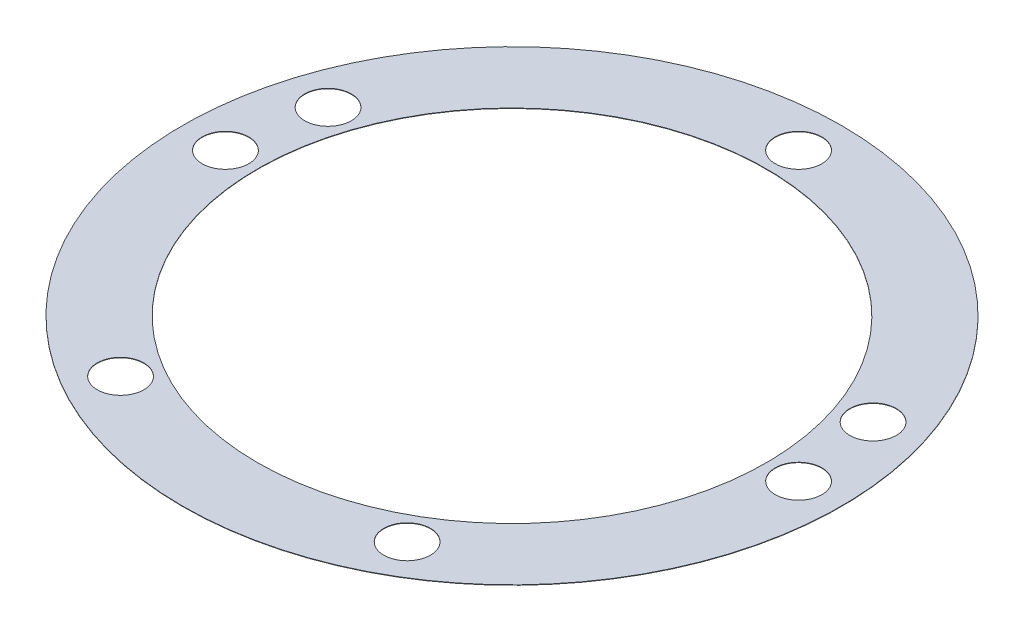
from build123d import *

# Parameters (mm, degrees)
SKETCH1_R                       = 146.05
SKETCH1_R_2                     = 112.776
BOSS_EXTRUDE1_DEPTH             = 0.1778
F_13_16_0_8125_DIAMETER_HOLE1_D = 20.6375
F_13_16_0_8125_DIAMETER_HOLE2_D = 20.6375


with BuildPart() as part:
    # Sketch1 → Boss-Extrude1 (new body)
    with BuildSketch(Plane(origin=(0, 0, 0), x_dir=(1, 0, 0), z_dir=(0, 1, 0))):
        with Locations(Location((0, 0, 0), (0, 0, 270))):
            Circle(SKETCH1_R)
        with Locations(Location((0, 0, 0), (0, 0, 270))):
            Circle(SKETCH1_R_2, mode=Mode.SUBTRACT)
    extrude(amount=BOSS_EXTRUDE1_DEPTH)

    # 13/16 (0.8125) Diameter Hole1 (through all)
    with Locations(Plane(origin=(0, 0.1778, 0), x_dir=(1, 0, 0), z_dir=(0, 1, 0))):
        with Locations((0, 127)):
            Hole(F_13_16_0_8125_DIAMETER_HOLE1_D / 2)

    # 13/16 (0.8125) Diameter Hole2 (through all)
    with Locations(Plane(origin=(0, 0, 0), x_dir=(-1, 0, 0), z_dir=(0, -1, 0))):
        with Locations((-63.5, -109.982), (-120.77, 39.243), (-127, 0)):
            f_13_16_0_8125_diameter_hole2 = Hole(F_13_16_0_8125_DIAMETER_HOLE2_D / 2)

    # Mirror1: 13/16 (0.8125) Diameter Hole2 across plane
    add(f_13_16_0_8125_diameter_hole2.mirror(Plane(origin=(0, 0, 0), x_dir=(0, 0, 1), z_dir=(1, 0, 0))), mode=Mode.SUBTRACT)


solid = part.part
